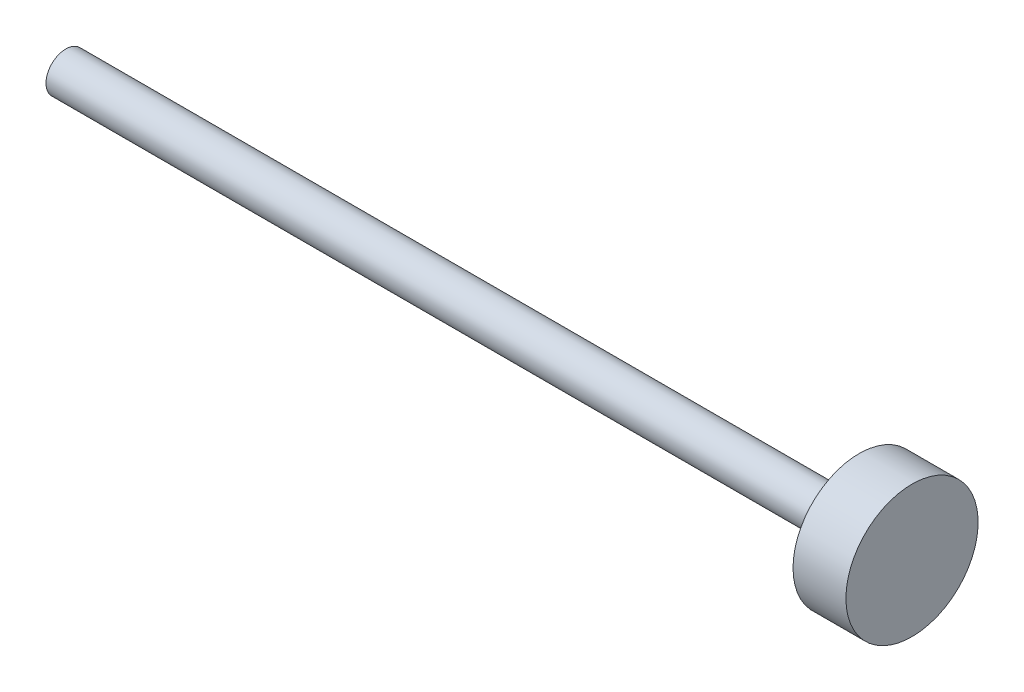
SolidWorks part; units mm, degrees
material "普通碳钢"
ref_plane "Front Plane" through (0, 0, 0) normal (0, 0, 1) x (1, 0, 0)
ref_plane "Top Plane" through (0, 0, 0) normal (0, 1, 0) x (1, 0, 0)
ref_plane "Right Plane" through (0, 0, 0) normal (1, 0, 0) x (0, 0, -1)
sketch "Sketch1" plane through (0, 0, 0) normal (0, 0, 1) x (1, 0, 0)
  line L0 (214.2204, 242.083) -> (534.2204, 242.083)
  line L1 (534.2204, 242.083) -> (534.2204, 267.083)
  line L2 (534.2204, 267.083) -> (514.2204, 267.083)
  line L3 (514.2204, 267.083) -> (514.2204, 249.583)
  line L4 (514.2204, 249.583) -> (214.2204, 249.583)
  line L5 (214.2204, 249.583) -> (214.2204, 242.083)
  dimension "D1" = 320
  dimension "D2" = 20
  dimension "D3" = 25
  dimension "D4" = 7.5
revolve "Revolve1" add sketch "Sketch1" angle 360 about L0
